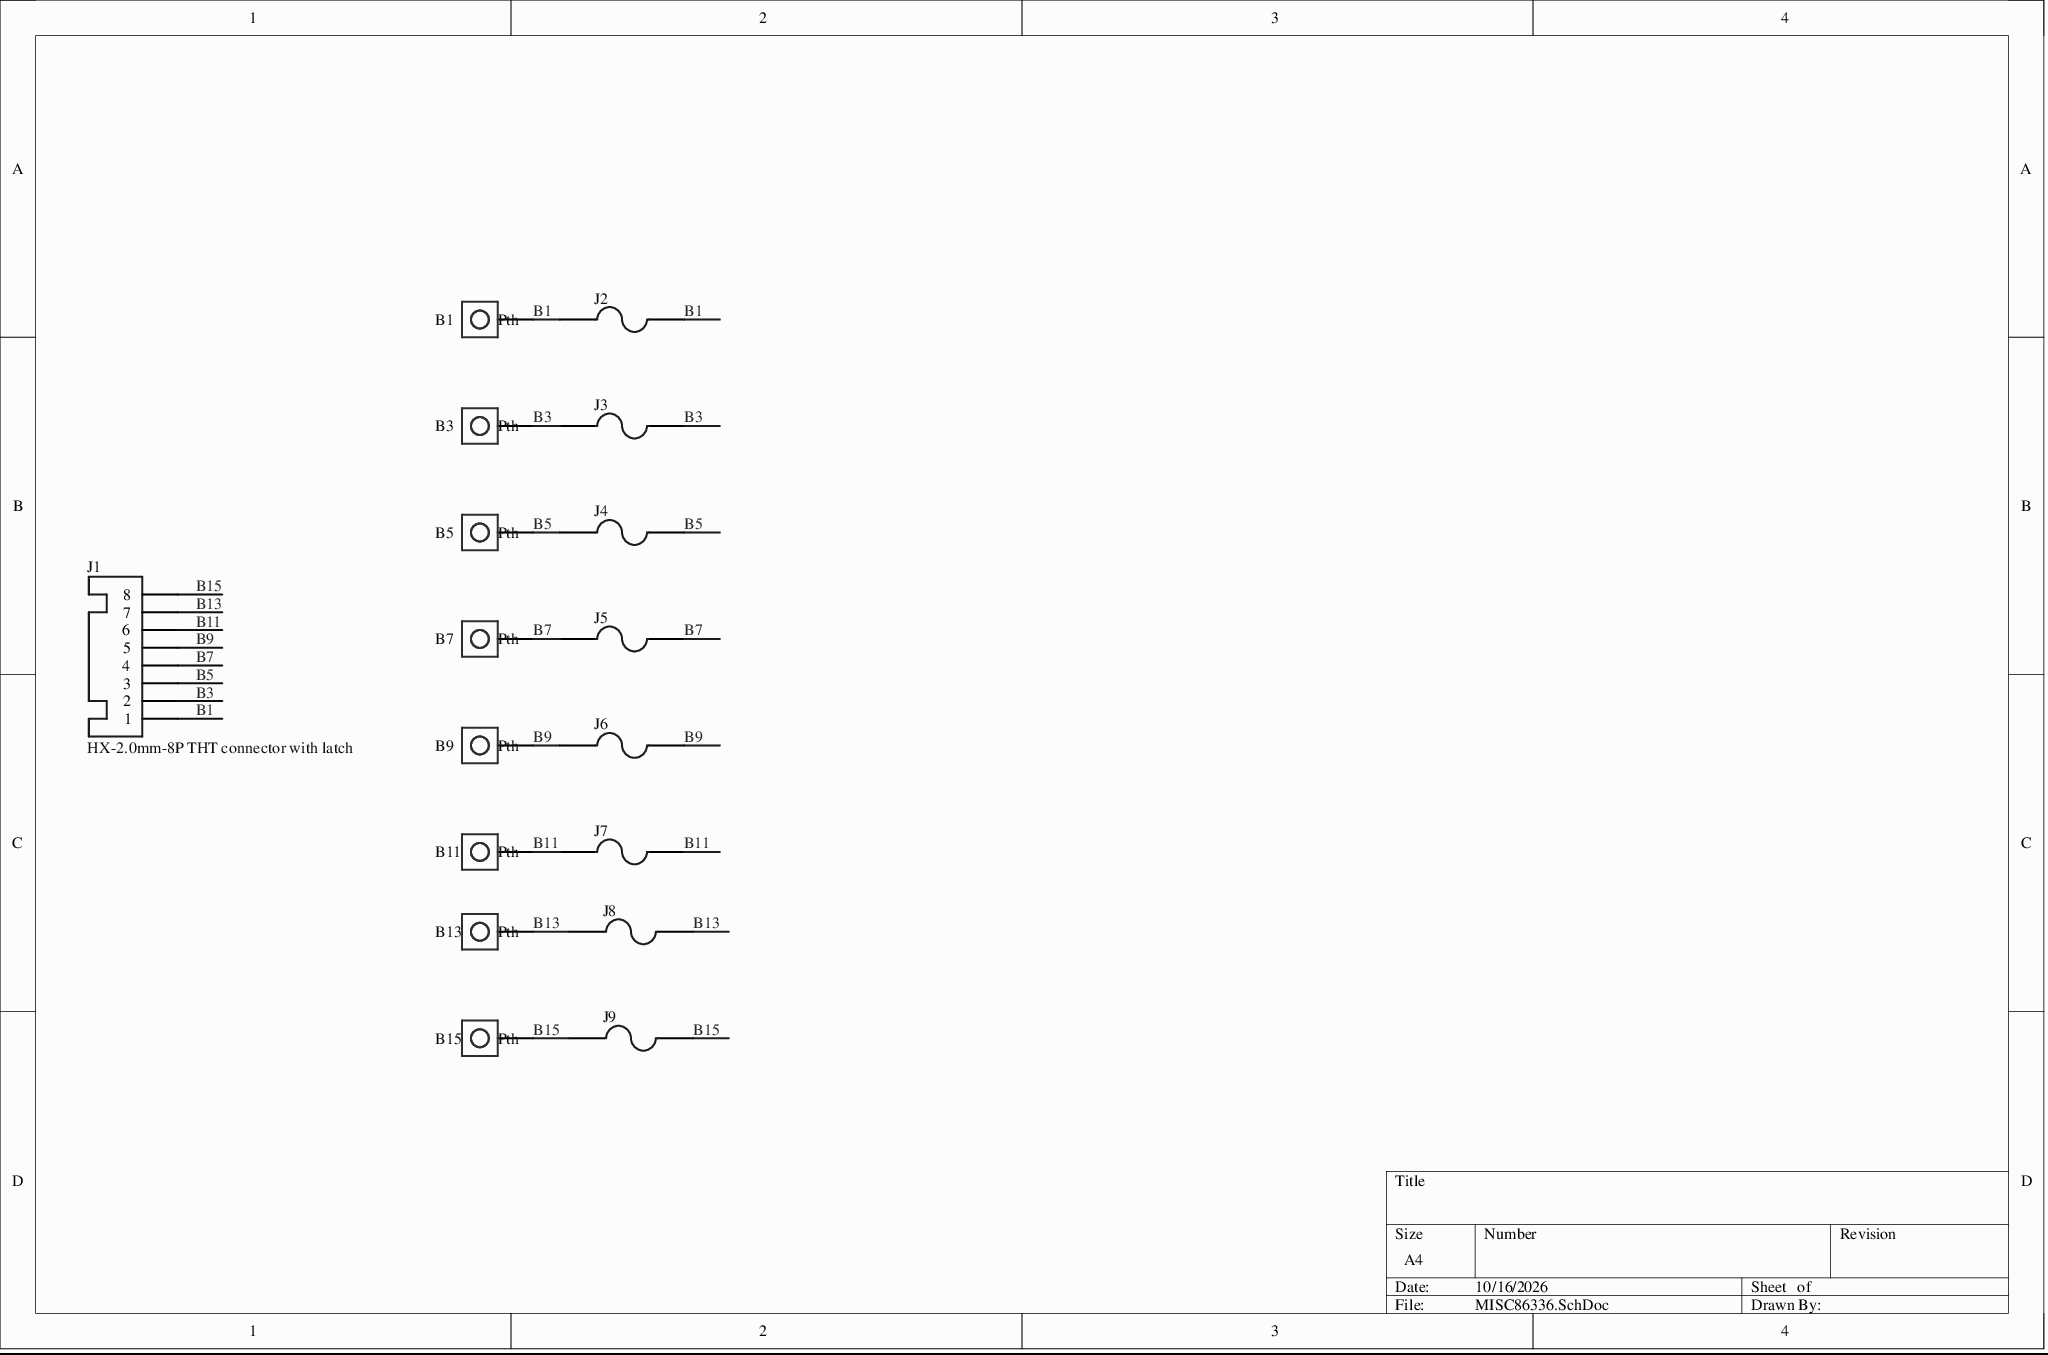
[diagram p0: MISC86336.SchDoc]
# Altium project MISC86336.PrjPcb
1 sheet, 17 parts. Net scope: global (net labels, ports and power ports of the same name join across sheets).
Board file: MISC86336.PcbDoc

## Sheet MISC86336.SchDoc
size A4; SheetNumber: 1; SheetTotal: 1

### Parts
B1  Pth  [55*10*1MM]
B3  Pth  [55*10*1MM]
B5  Pth  [55*10*1MM]
B7  Pth  [55*10*1MM]
B9  Pth  [55*10*1MM]
B11  Pth  [55*10*1MM]
B13  Pth  [55*10*1MM]
B15  Pth  [55*10*1MM]
J1  HX-2.0mm-8P THT connector with latch  [HX2.0-8P]
J2  FPC  [异形电阻]  (value not drawn)
J3  FPC  [异形电阻]  (value not drawn)
J4  FPC  [异形电阻]  (value not drawn)
J5  FPC  [异形电阻]  (value not drawn)
J6  FPC  [异形电阻]  (value not drawn)
J7  FPC  [异形电阻]  (value not drawn)
J8  FPC  [异形电阻]  (value not drawn)
J9  FPC  [异形电阻]  (value not drawn)

### Nets
B1: B1.1 J1.1 J2.1 J2.2
B3: B3.1 J1.2 J3.1 J3.2
B5: B5.1 J1.3 J4.1 J4.2
B7: B7.1 J1.4 J5.1 J5.2
B9: B9.1 J1.5 J6.1 J6.2
B11: B11.1 J1.6 J7.1 J7.2
B13: B13.1 J1.7 J8.1 J8.2
B15: B15.1 J1.8 J9.1 J9.2

### Library data of the parts
B1 B3 B5 B7 B9 B11 B13 B15 = Pth: Through-hole pad
J1 = HX-2.0mm-8P直插带扣